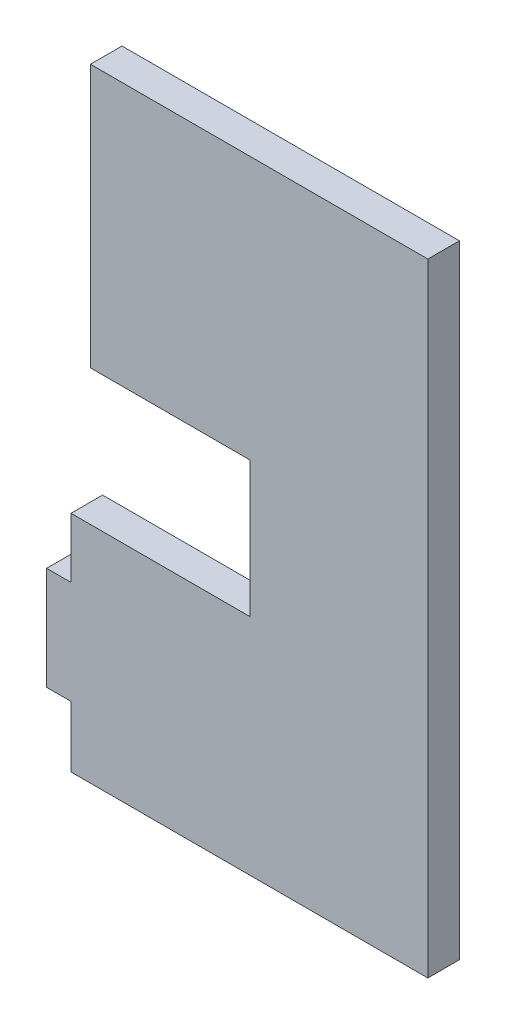
SolidWorks part; units mm, degrees
ref_plane "Front Plane" through (0, 0, 0) normal (0, 0, 1) x (1, 0, 0)
ref_plane "Top Plane" through (0, 0, 0) normal (0, 1, 0) x (1, 0, 0)
ref_plane "Right Plane" through (0, 0, 0) normal (1, 0, 0) x (0, 0, -1)
sketch "Sketch1" plane through (0, 0, 0) normal (0, 0, 1) x (1, 0, 0)
  line L0 (3, -18.5843) -> (0.6808, -18.5843)
  line L2 (0.6808, -18.5843) -> (0.6808, -28.3851)
  line L3 (0.6808, -28.3851) -> (3, -28.3851)
  line L4 (3, -28.3851) -> (3, -34.193)
  line L5 (3, -34.193) -> (36.9231, -34.193)
  line L6 (3, -18.5843) -> (3, -12.8946)
  line L7 (3, -12.8946) -> (20, -12.8946)
  line L9 (20, -12.8946) -> (20, 0)
  line L10 (20, 0) -> (4.8471, 0)
  line L12 (4.8471, 0) -> (4.8471, 25)
  line L13 (4.8471, 25) -> (36.9231, 25)
  line L14 (36.9231, 25) -> (36.9231, -34.193)
  dimension "D1" = 25
extrude "Boss-Extrude1" add sketch "Sketch1" along normal blind 3
